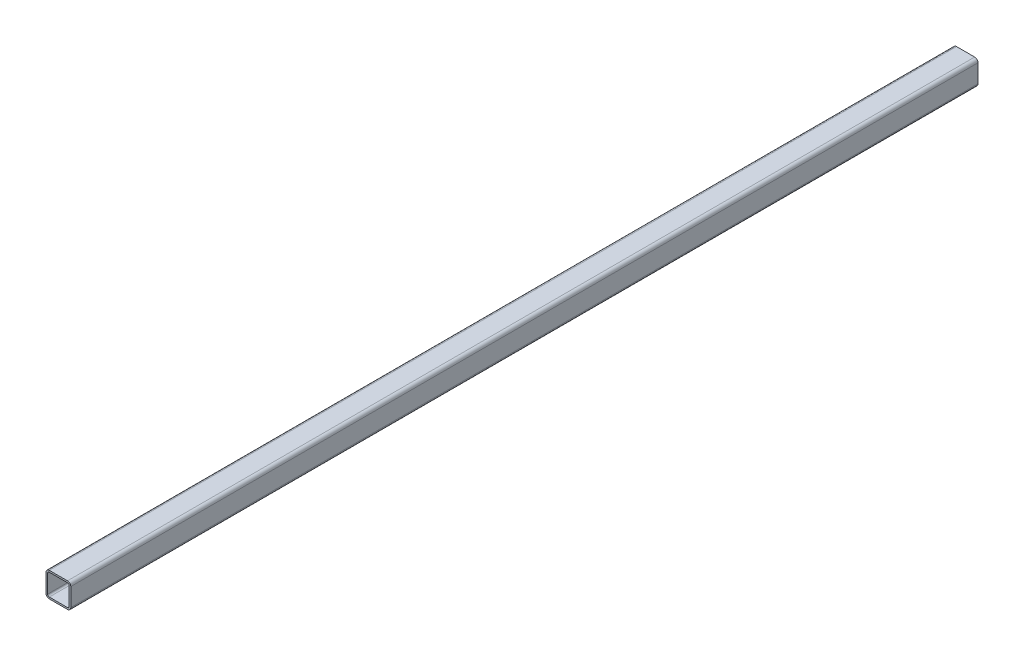
from build123d import *

# Parameters (mm, degrees)
EXTRUDE_THIN1_DEPTH = 548.8


with BuildPart() as part:
    # Sketch1 → Extrude-Thin1 (new, symmetric)
    with BuildSketch(Plane.XY):
        with BuildLine():
            Line((-15, 11), (-15, -11))
            ThreePointArc((-15, -11), (-13.828427125, -13.828427125), (-11, -15))
            Line((-11, -15), (11, -15))
            ThreePointArc((11, -15), (13.828427125, -13.828427125), (15, -11))
            Line((15, -11), (15, 11))
            ThreePointArc((15, 11), (13.828427125, 13.828427125), (11, 15))
            Line((11, 15), (-11, 15))
            ThreePointArc((-11, 15), (-13.828427125, 13.828427125), (-15, 11))
        make_face()
        with BuildLine():
            Line((-13, 11), (-13, -11))
            ThreePointArc((-13, -11), (-12.414213562, -12.414213562), (-11, -13))
            Line((-11, -13), (11, -13))
            ThreePointArc((11, -13), (12.414213562, -12.414213562), (13, -11))
            Line((13, -11), (13, 11))
            ThreePointArc((13, 11), (12.414213562, 12.414213562), (11, 13))
            Line((11, 13), (-11, 13))
            ThreePointArc((-11, 13), (-12.414213562, 12.414213562), (-13, 11))
        make_face(mode=Mode.SUBTRACT)
    extrude(amount=EXTRUDE_THIN1_DEPTH, both=True)


solid = part.part
